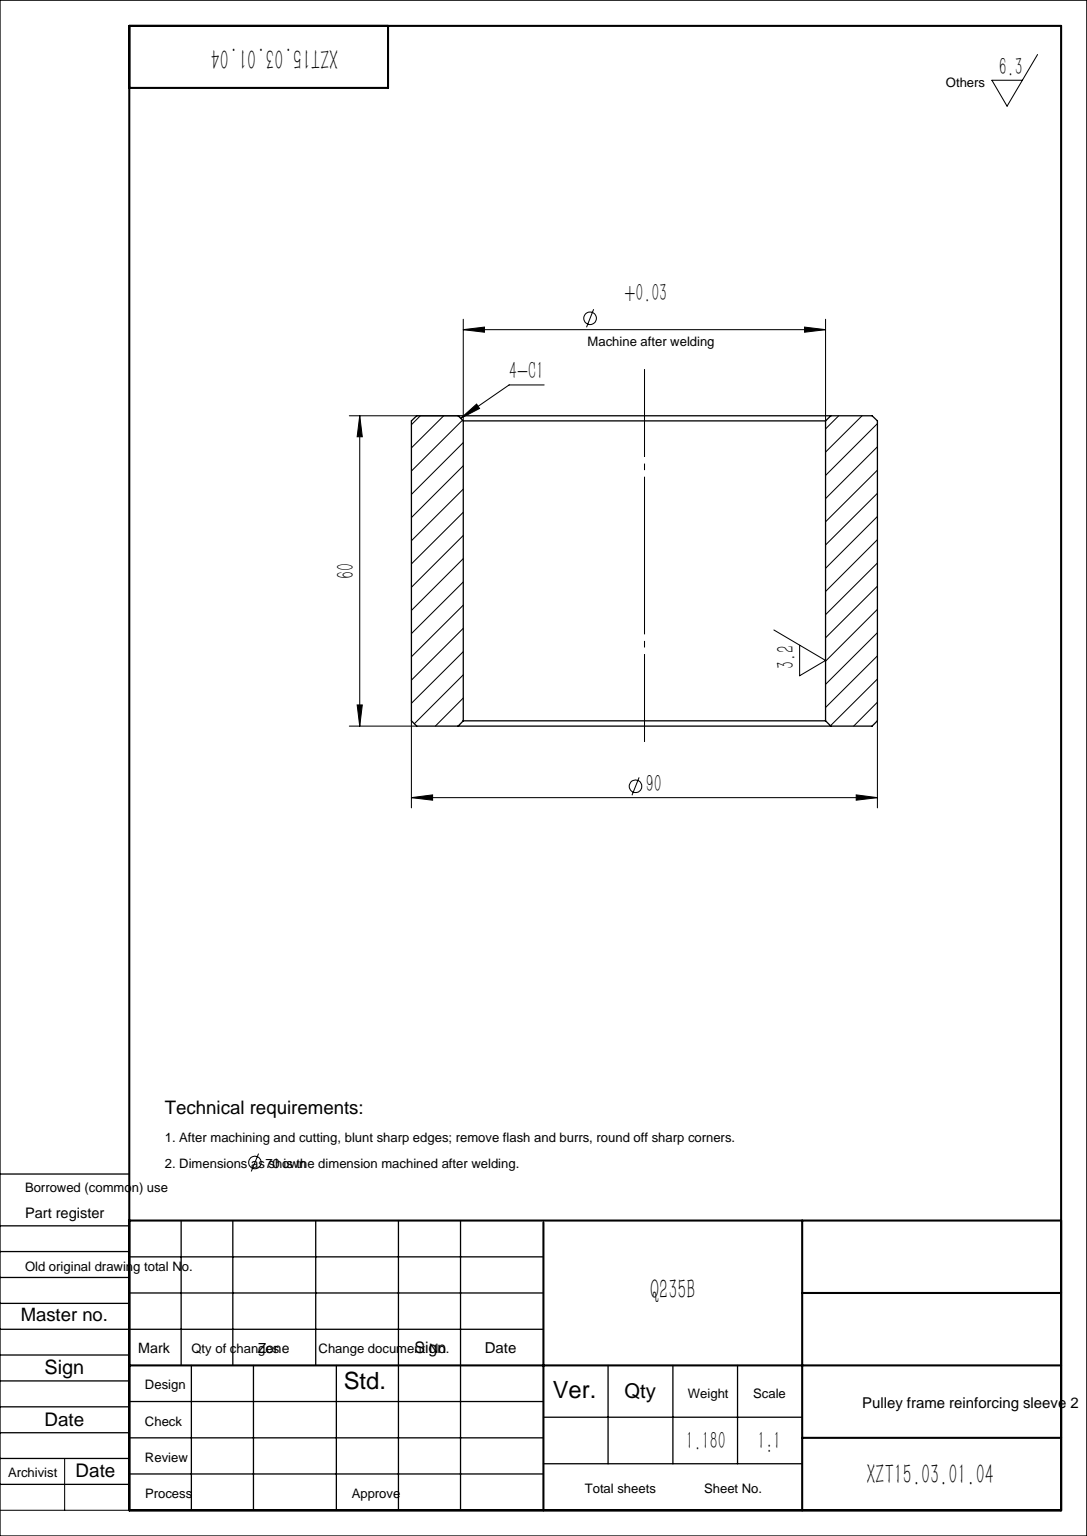
from build123d import *

# Parameters (mm, degrees)
SKETCH1_R           = 45
SKETCH1_R_2         = 35
BOSS_EXTRUDE1_DEPTH = 60
CHAMFER2_SIZE       = 1


with BuildPart() as part:
    # Sketch1 → Boss-Extrude1 (new body)
    with BuildSketch(Plane(origin=(0, 0, 0), x_dir=(1, 0, 0), z_dir=(0, 1, 0))):
        with Locations(Location((0, 0, 0), (0, 0, 270))):
            Circle(SKETCH1_R)
        with Locations(Location((0, 0, 0), (0, 0, 270))):
            Circle(SKETCH1_R_2, mode=Mode.SUBTRACT)
    extrude(amount=BOSS_EXTRUDE1_DEPTH)

    # Chamfer2
    chamfer2_edges = [part.edges().sort_by_distance(p)[0] for p in [
        (0, 0, -45),
        (0, 60, -45),
        (0, 0, -35),
        (0, 60, -35),
    ]]
    chamfer(chamfer2_edges, length=CHAMFER2_SIZE)


solid = part.part
